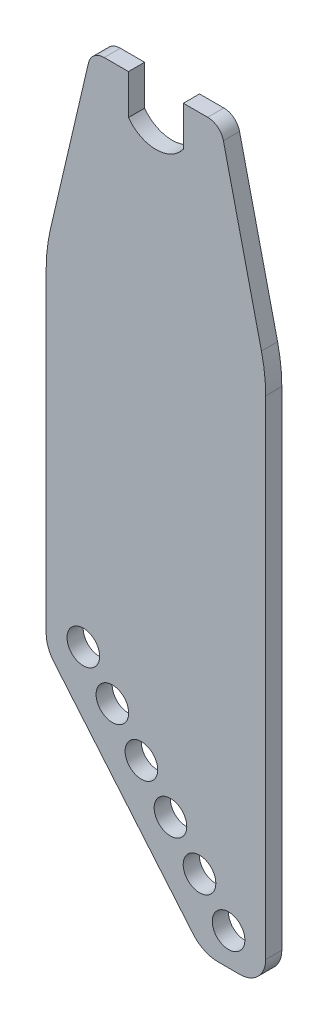
from build123d import *

# Parameters (mm, degrees)
SKETCH1_W           = 68
SKETCH1_H           = 225
BOSS_EXTRUDE1_DEPTH = 5
SKETCH3_R           = 5.05
CUT_EXTRUDE1_DEPTH  = 8
FILLET1_R           = 8
CUT_EXTRUDE2_DEPTH  = 118.631840928
FILLET2_R           = 10
CUT_EXTRUDE3_DEPTH  = 8
FILLET3_R           = 10
CUT_EXTRUDE4_DEPTH  = 118.631840928
FILLET4_R           = 5
FILLET5_R           = 50


with BuildPart() as part:
    # Sketch1 → Boss-Extrude1 (new body)
    with BuildSketch(Plane.XY):
        Rectangle(SKETCH1_W, SKETCH1_H)
    extrude(amount=BOSS_EXTRUDE1_DEPTH)

    # Sketch3 → Cut-Extrude1 (cut)
    with BuildSketch(Plane.XY.offset(5)):
        with Locations((22.5, -102.5)):
            Circle(SKETCH3_R)
        with Locations((13.500973464, -91.775377796)):
            Circle(SKETCH3_R)
        with Locations((4.501946929, -81.050755593)):
            Circle(SKETCH3_R)
        with Locations((-4.497079607, -70.326133389)):
            Circle(SKETCH3_R)
        with Locations((-13.496106142, -59.601511185)):
            Circle(SKETCH3_R)
        with Locations((-22.495132678, -48.876888982)):
            Circle(SKETCH3_R)
    extrude(amount=-CUT_EXTRUDE1_DEPTH, mode=Mode.SUBTRACT)

    # Fillet1
    fillet1_edges = [part.edges().sort_by_distance(p)[0] for p in [
        (34, -112.5, 2.5),
    ]]
    fillet(fillet1_edges, radius=FILLET1_R)

    # Sketch5 → Cut-Extrude2 (cut, through all)
    with BuildSketch(Plane.XY.offset(5)):
        Polygon((14.573405195, -112.5), (-34, -54.612469854), (-34, -112.5), align=None)
    extrude(amount=-CUT_EXTRUDE2_DEPTH, mode=Mode.SUBTRACT)

    # Fillet2
    fillet2_edges = [part.edges().sort_by_distance(p)[0] for p in [
        (14.573405195, -112.5, 2.5),
    ]]
    fillet(fillet2_edges, radius=FILLET2_R)

    # Sketch6 → Cut-Extrude3 (cut)
    with BuildSketch(Plane.XY.offset(5)):
        with BuildLine():
            Line((-8.5, 112.5), (-8.5, 100.171171994))
            ThreePointArc((-8.5, 100.171171994), (0, 95.835585997), (8.5, 100.171171994))
            Line((8.5, 100.171171994), (8.5, 112.5))
            ThreePointArc((8.5, 112.5), (0, 116.835585997), (-8.5, 112.5))
        make_face()
    extrude(amount=-CUT_EXTRUDE3_DEPTH, mode=Mode.SUBTRACT)

    # Fillet3
    fillet3_edges = [part.edges().sort_by_distance(p)[0] for p in [
        (-34, -54.612469854, 2.5),
    ]]
    fillet(fillet3_edges, radius=FILLET3_R)

    # Sketch7 → Cut-Extrude4 (cut, through all)
    with BuildSketch(Plane.XY.offset(5)):
        Polygon((-20, 112.5), (-34, 52.5), (-34, 112.5), align=None)
        Polygon((34, 112.5), (20, 112.5), (34, 52.5), align=None)
    extrude(amount=-CUT_EXTRUDE4_DEPTH, mode=Mode.SUBTRACT)

    # Fillet4
    fillet4_edges = [part.edges().sort_by_distance(p)[0] for p in [
        (-20, 112.5, 2.5),
        (20, 112.5, 2.5),
    ]]
    fillet(fillet4_edges, radius=FILLET4_R)

    # Fillet5
    fillet5_edges = [part.edges().sort_by_distance(p)[0] for p in [
        (-34, 52.5, 2.5),
        (34, 52.5, 2.5),
    ]]
    fillet(fillet5_edges, radius=FILLET5_R)


solid = part.part
